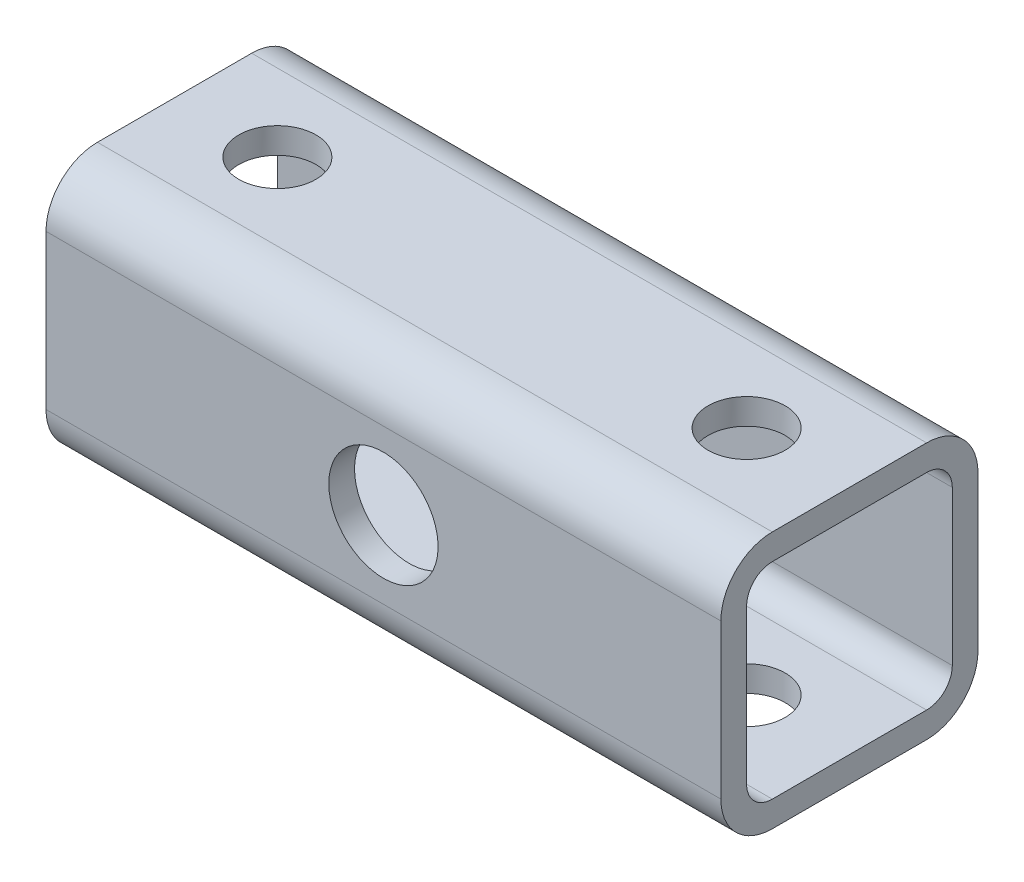
from build123d import *

# Parameters (mm, degrees)
GB_T6728_2002_40_X_40_X_4_1_DEPTH = 105
HOLE_WIZARD_12_0_12_1_D           = 12
HOLE_WIZARD_12_0_12_1_DEPTH       = 41.394836286
HOLE_WIZARD_12_0_12_1_TIP         = 3.605163714
CUT_EXTRUDE_1_REACH               = 116.127
SKETCH_5_R                        = 8.5


with BuildPart() as part:
    # Sketch1 → 冷弯空心方管gb∕t6728-2002 40 X 40 X 4(1) (new body)
    with BuildSketch(Plane.YZ):
        with BuildLine():
            Line((-12, -20), (12, -20))
            ThreePointArc((12, -20), (17.656854249, -17.656854249), (20, -12))
            Line((20, -12), (20, 12))
            ThreePointArc((20, 12), (17.656854249, 17.656854249), (12, 20))
            Line((12, 20), (-12, 20))
            ThreePointArc((-12, 20), (-17.656854249, 17.656854249), (-20, 12))
            Line((-20, 12), (-20, -12))
            ThreePointArc((-20, -12), (-17.656854249, -17.656854249), (-12, -20))
        make_face()
        with BuildLine():
            Line((-12, -16), (12, -16))
            ThreePointArc((12, -16), (14.828427125, -14.828427125), (16, -12))
            Line((16, -12), (16, 12))
            ThreePointArc((16, 12), (14.828427125, 14.828427125), (12, 16))
            Line((12, 16), (-12, 16))
            ThreePointArc((-12, 16), (-14.828427125, 14.828427125), (-16, 12))
            Line((-16, 12), (-16, -12))
            ThreePointArc((-16, -12), (-14.828427125, -14.828427125), (-12, -16))
        make_face(mode=Mode.SUBTRACT)
    extrude(amount=GB_T6728_2002_40_X_40_X_4_1_DEPTH)

    # Ø12.0 (12) 直径孔1
    with Locations(Plane(origin=(0, 20, 0), x_dir=(1, 0, 0), z_dir=(0, 1, 0))):
        with Locations((16, 0), (89, 0)):
            Hole(HOLE_WIZARD_12_0_12_1_D / 2, depth=HOLE_WIZARD_12_0_12_1_DEPTH)
            with Locations((0, 0, -(HOLE_WIZARD_12_0_12_1_DEPTH + HOLE_WIZARD_12_0_12_1_TIP / 2))):  # 118° drill point
                Cone(0, HOLE_WIZARD_12_0_12_1_D / 2, HOLE_WIZARD_12_0_12_1_TIP, mode=Mode.SUBTRACT)

    # 切除-拉伸1: up to this face of the body (flat: up to its plane)
    cut_extrude_1_end = Plane(part.part.faces().sort_by_distance((52.5, 0, 20))[0])
    # 草图5 → 切除-拉伸1 (cut, up to the picked face)
    with BuildSketch(Plane(origin=(0, 0, -20), x_dir=(-1, 0, 0), z_dir=(0, 0, -1)), mode=Mode.PRIVATE) as cut_extrude_1_sk1:
        with Locations((-52.5, 0)):
            Circle(SKETCH_5_R)
    cut_extrude_1_tool1 = split(extrude(cut_extrude_1_sk1.sketch, amount=-CUT_EXTRUDE_1_REACH, mode=Mode.PRIVATE), bisect_by=cut_extrude_1_end, keep=Keep.BOTH, mode=Mode.PRIVATE)
    add(cut_extrude_1_tool1.solids().sort_by(Axis((52.5, 0, -20), (0, 0, 1)))[0], mode=Mode.SUBTRACT)


solid = part.part
